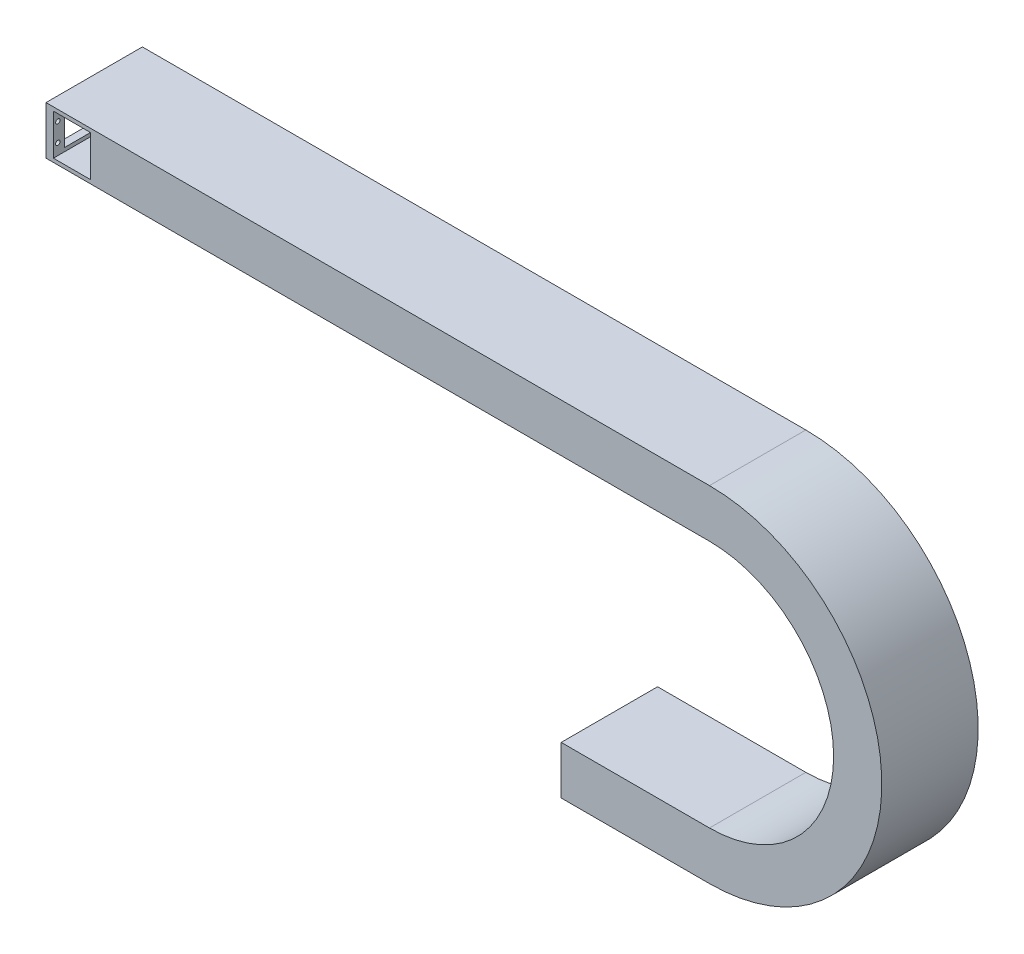
from build123d import *

# Parameters (mm, degrees)
EXTRUDE_1_DEPTH     = 130
SKETCH_2_R          = 3
CUT_EXTRUDE_1_DEPTH = 20
SKETCH_9_W          = 50
SKETCH_9_H          = 55
CUT_EXTRUDE_2_DEPTH = 150
SKETCH_10_W         = 100
SKETCH_10_H         = 45
CUT_EXTRUDE_3_DEPTH = 200


with BuildPart() as part:
    # 草图1 → 凸台-拉伸1 (new body)
    with BuildSketch(Plane.XY):
        with BuildLine():
            Line((-5035.427662897, 234.022122697), (-5930.427662897, 234.022122697))
            Line((-5930.427662897, 234.022122697), (-5930.427662897, 299.022122697))
            Line((-5930.427662897, 299.022122697), (-5035.427662897, 299.022122697))
            ThreePointArc((-5035.427662897, 299.022122697), (-4802.927662897, 66.522122697), (-5035.427662897, -165.977877303))
            Line((-5035.427662897, -165.977877303), (-5235.427662897, -165.977877303))
            Line((-5235.427662897, -165.977877303), (-5235.427662897, -100.977877303))
            Line((-5235.427662897, -100.977877303), (-5035.427662897, -100.977877303))
            ThreePointArc((-5035.427662897, -100.977877303), (-4867.927662897, 66.522122697), (-5035.427662897, 234.022122697))
        make_face()
    extrude(amount=EXTRUDE_1_DEPTH)

    # 草图2 → 切除-拉伸1 (cut)
    with BuildSketch(Plane.ZY.offset(5930.427662897)):
        with Locations((6, 279.022122697)):
            Circle(SKETCH_2_R)
        with Locations((6, 254.022122697)):
            Circle(SKETCH_2_R)
        with Locations((124, 279.022122697)):
            Circle(SKETCH_2_R)
        with Locations((124, 254.022122697)):
            Circle(SKETCH_2_R)
    extrude(amount=-CUT_EXTRUDE_1_DEPTH, mode=Mode.SUBTRACT)

    # 草图9 → 切除-拉伸2 (cut)
    with BuildSketch(Plane.XY.offset(130)):
        with Locations((-5895.427662897, 266.522122697)):
            Rectangle(SKETCH_9_W, SKETCH_9_H)
    extrude(amount=-CUT_EXTRUDE_2_DEPTH, mode=Mode.SUBTRACT)

    # 草图10 → 切除-拉伸3 (cut)
    with BuildSketch(Plane.ZY.offset(5930.427662897)):
        with Locations((65, 266.522122697)):
            Rectangle(SKETCH_10_W, SKETCH_10_H)
    extrude(amount=-CUT_EXTRUDE_3_DEPTH, mode=Mode.SUBTRACT)


solid = part.part
